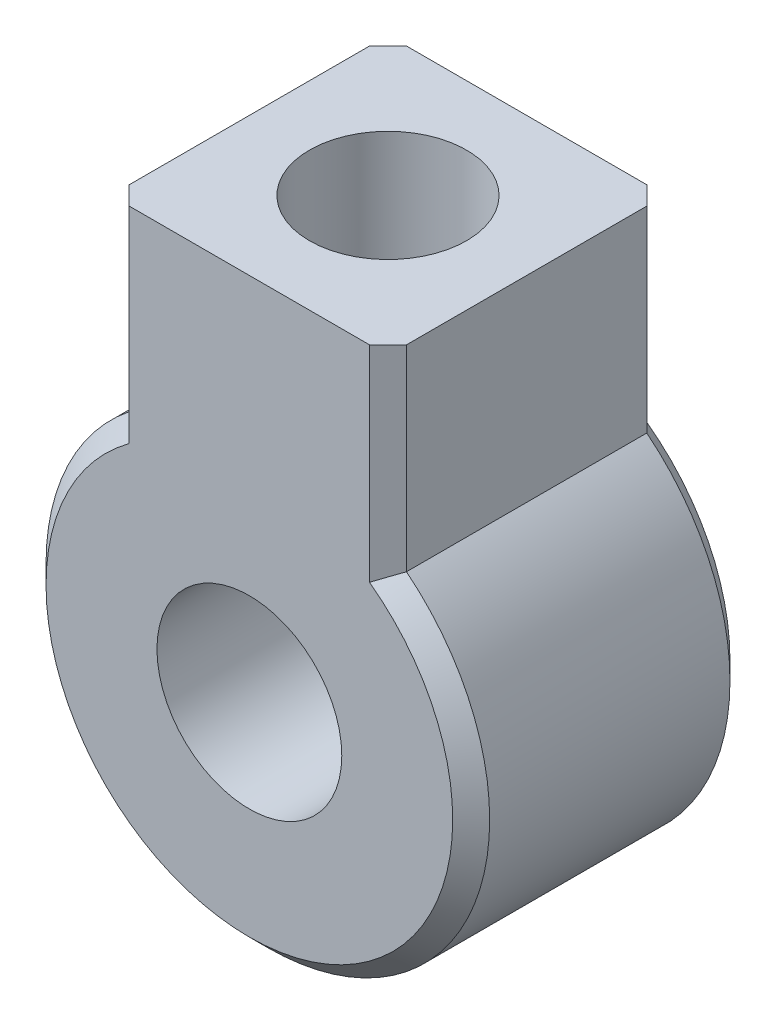
SolidWorks part; units mm, degrees
ref_plane "前视基准面" through (0, 0, 0) normal (0, 0, 1) x (1, 0, 0)
ref_plane "上视基准面" through (0, 0, 0) normal (0, 1, 0) x (1, 0, 0)
ref_plane "右视基准面" through (0, 0, 0) normal (1, 0, 0) x (0, 0, -1)
ref_plane "基准面4" through (0, 0, 7.5) normal (0, 0, 1) x (1, 0, 0)
sketch "草图1" plane through (0, 0, 7.5) normal (0, 0, 1) x (1, 0, 0)
  line L0 (7.5, 20) -> (-7.5, 20)
  line L1 (-7.5, 20) -> (-7.5, 9.3675)
  line L2 (7.5, 9.3675) -> (7.5, 20)
  arc A0 (-7.5, 9.3675) -> (7.5, 9.3675) centre (0, 0) ccw
extrude "凸台-拉伸1" add sketch "草图1" against normal blind 15
hole_wizard "Ø10.0 (10) 直径孔1" positions "草图3" profile "草图2" hole size "Ø10.0" standard "ANSI Metric"
sketch "草图3" plane through (0, 0, 7.5) normal (0, 0, 1) x (1, 0, 0)
  point P0 (0, 0)
sketch "草图2" plane through (0, 0, 7.5) normal (1, 0, 0) x (0, -1, 0)
  line L0 (0, 0) -> (0, 15)
  line L1 (0, 15) -> (5, 15)
  line L2 (5, 15) -> (5, 0)
  line L5 (5, 0) -> (0, 0)
  line L11 (0, -6.35) -> (0, 107.95) construction
  dimension "通孔孔直径" = 10
  dimension "通孔孔深度" = 15
hole_wizard "Ø8.5 (8.5) 直径孔1" positions "草图5" profile "草图4" hole size "Ø8.5" standard "ANSI Metric"
sketch "草图5" plane through (0, 20, 0) normal (0, 1, 0) x (1, 0, 0)
  point P0 (0, 0)
sketch "草图4" plane through (0, 20, 0) normal (1, 0, 0) x (0, 0, 1)
  line L0 (0, 0) -> (0, 15)
  line L1 (0, 15) -> (4.25, 15)
  line L2 (4.25, 15) -> (4.25, 0)
  line L5 (4.25, 0) -> (0, 0)
  line L11 (0, -6.35) -> (0, 107.95) construction
  dimension "通孔孔直径" = 8.5
  dimension "通孔孔深度" = 15
chamfer "倒角1" distance 1 angle 45 6 edges at (7.5, 14.6837, -7.5) (0, -12, -7.5) (-7.5, 14.6837, -7.5) (7.5, 14.6837, 7.5) (-7.5, 14.6837, 7.5) (0, -12, 7.5)
